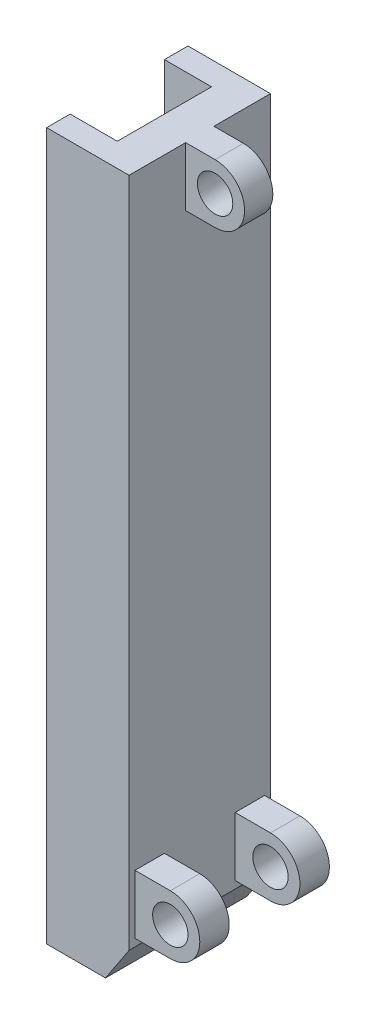
from build123d import *

# Parameters (mm, degrees)
BOSS_EXTRUDE1_DEPTH      = 600
SKETCH2_R                = 15
BOSS_EXTRUDE2_DEPTH      = 30
BOSS_EXTRUDE3_DEPTH      = 12
BOSS_EXTRUDE3_DEPTH_BACK = 12
SKETCH3_R                = 15
SKETCH4_W                = 64.999273694
SKETCH4_H                = 54.968001075
CUT_EXTRUDE1_DEPTH       = 5
CUT_EXTRUDE2_DEPTH       = 621.826062597


with BuildPart() as part:
    # Sketch1 → Boss-Extrude1 (new body)
    with BuildSketch(Plane(origin=(0, 0, 0), x_dir=(1, 0, 0), z_dir=(0, 1, 0))):
        Polygon((-20, 40), (-20, 60), (50, 60), (50, -60), (-20, -60), (-20, -40), (20, -40), (20, 40), align=None)
    extrude(amount=BOSS_EXTRUDE1_DEPTH)

    # Sketch2 → Boss-Extrude2 (add)
    with BuildSketch(Plane(origin=(0, 0, -60), x_dir=(-1, 0, 0), z_dir=(0, 0, -1))):
        with BuildLine():
            Line((-34.984231122, 36.653571932), (-80, 36.653571932))
            ThreePointArc((-80, 36.653571932), (-105, 61.653571932), (-80, 86.653571932))
            Line((-80, 86.653571932), (-34.984231122, 86.653571932))
            Line((-34.984231122, 86.653571932), (-34.984231122, 36.653571932))
        make_face()
        with Locations((-80, 61.653571932)):
            Circle(SKETCH2_R, mode=Mode.SUBTRACT)
    boss_extrude2 = extrude(amount=-BOSS_EXTRUDE2_DEPTH)

    # Mirror1: Boss-Extrude2 across plane
    add(boss_extrude2.mirror(Plane.XY))

    # Sketch3 → Boss-Extrude3 (add, two sides: drawn at the far end of the back side and taken through both)
    with BuildSketch(Plane.XY.offset(-BOSS_EXTRUDE3_DEPTH_BACK)):
        with BuildLine():
            Line((42.373646318, 600), (75, 600))
            ThreePointArc((75, 600), (100, 575), (75, 550))
            Line((75, 550), (42.373646318, 550))
            Line((42.373646318, 550), (42.373646318, 600))
        make_face()
        with Locations((75, 575)):
            Circle(SKETCH3_R, mode=Mode.SUBTRACT)
    extrude(amount=BOSS_EXTRUDE3_DEPTH + BOSS_EXTRUDE3_DEPTH_BACK)

    # Sketch4 → Cut-Extrude1 (cut)
    with BuildSketch(Plane(origin=(0, 0, -60), x_dir=(-1, 0, 0), z_dir=(0, 0, -1))):
        with Locations((-82.499636847, 64.13757247)):
            Rectangle(SKETCH4_W, SKETCH4_H)
    cut_extrude1 = extrude(amount=-CUT_EXTRUDE1_DEPTH, mode=Mode.SUBTRACT)

    # Mirror2: Cut-Extrude1 across plane
    add(cut_extrude1.mirror(Plane.XY), mode=Mode.SUBTRACT)

    # Sketch5 → Cut-Extrude2 (cut, through all)
    with BuildSketch(Plane(origin=(0, 0, -60), x_dir=(-1, 0, 0), z_dir=(0, 0, -1))):
        Polygon((-50, 30.340627067), (-30, 0), (-50, 0), align=None)
    extrude(amount=-CUT_EXTRUDE2_DEPTH, mode=Mode.SUBTRACT)


solid = part.part
